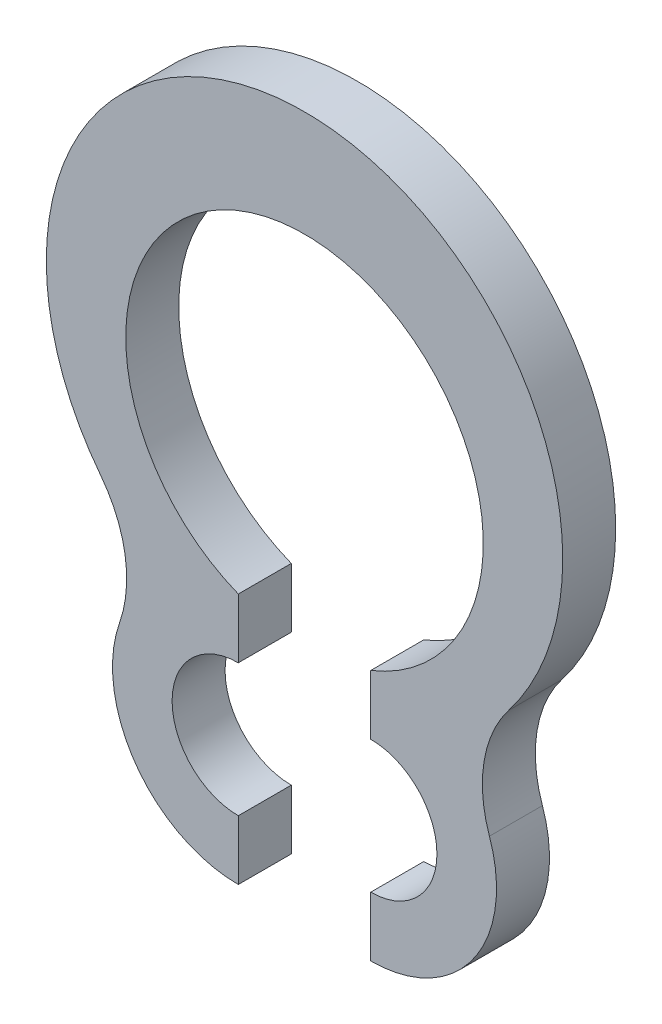
SolidWorks part; units mm, degrees
ref_plane "Front" through (0, 0, 0) normal (0, 0, 1) x (1, 0, 0)
ref_plane "Top" through (0, 0, 0) normal (0, 1, 0) x (1, 0, 0)
ref_plane "Right" through (0, 0, 0) normal (1, 0, 0) x (0, 0, -1)
other "Configuration Table"
sketch "Sketch1" plane through (0, 0, 0) normal (0, 0, 1) x (1, 0, 0)
  line L0 (0, -0.2) -> (0, -3.1859) construction
  line L1 (-0.5, -1.454) -> (-0.5, -1.904)
  line L2 (-0.5, -2.904) -> (-0.5, -3.354)
  line L3 (0.5, -2.904) -> (0.5, -3.354)
  line L4 (0.5, -1.454) -> (0.5, -1.904)
  arc A0 (0.5, -1.454) -> (-0.5, -1.454) centre (0, -0.2) ccw
  arc A1 (1.5419, -1.1938) -> (-1.5419, -1.1938) centre (0, 0) ccw
  arc A2 (-0.5, -1.904) -> (-0.5, -2.904) centre (-0.5, -2.404) ccw
  arc A3 (-0.5, -3.354) -> (-1.3965, -2.0897) centre (-0.5, -2.404) cw
  arc A4 (-1.5419, -1.1938) -> (-1.3965, -2.0897) centre (-2.293, -1.7754) cw
  arc A5 (1.5419, -1.1938) -> (1.3965, -2.0897) centre (2.293, -1.7754) ccw
  arc A6 (0.5, -3.354) -> (1.3965, -2.0897) centre (0.5, -2.404) ccw
  arc A7 (0.5, -1.904) -> (0.5, -2.904) centre (0.5, -2.404) cw
extrude "Body" add sketch "Sketch1" against normal blind 0.4 separate body
equation "\"D2@Sketch1\" = \"d1@Sketch1\""
equation "\"R3@Sketch1\" = \"h@Sketch1\""
